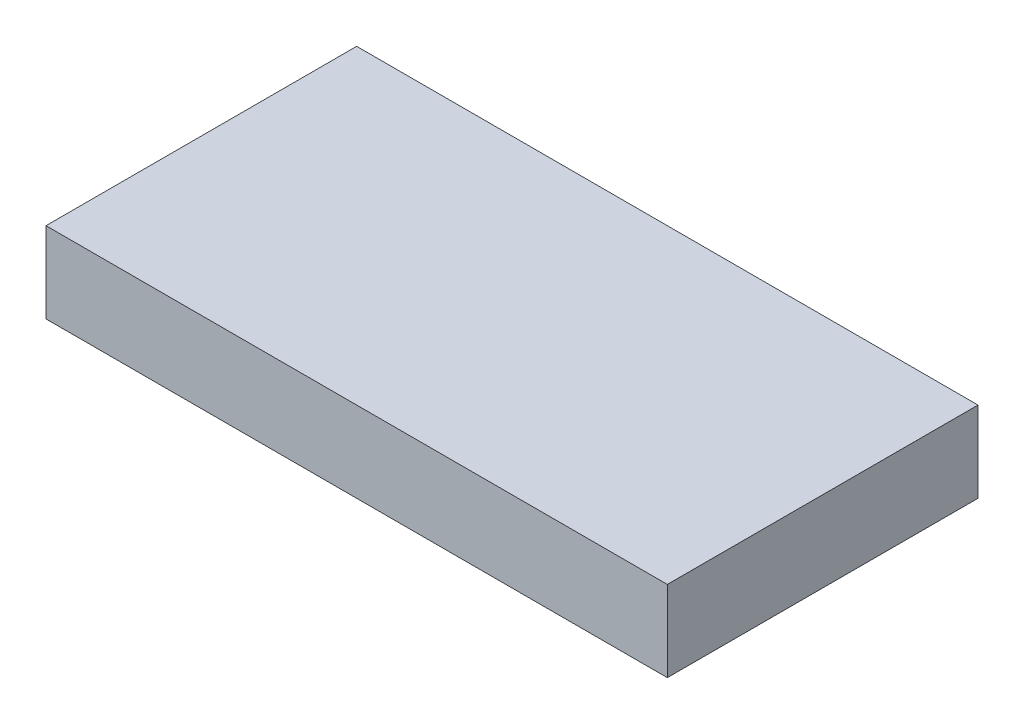
SolidWorks part; units mm, degrees
ref_plane "Front Plane" through (0, 0, 0) normal (0, 0, 1) x (1, 0, 0)
ref_plane "Top Plane" through (0, 0, 0) normal (0, 1, 0) x (1, 0, 0)
ref_plane "Right Plane" through (0, 0, 0) normal (1, 0, 0) x (0, 0, -1)
sketch "Sketch1" plane through (0, 0, 0) normal (0, 1, 0) x (1, 0, 0)
  line L1 (-10, 5) -> (10, 5)
  line L2 (-10, 5) -> (-10, -5)
  line L3 (-10, -5) -> (10, -5)
  line L4 (10, 5) -> (10, -5)
  line L5 (-10, 5) -> (10, -5) construction
  line L6 (-10, -5) -> (10, 5) construction
  point P0 (0, 0)
  dimension "D1" = 10
  dimension "D2" = 20
extrude "Boss-Extrude1" add sketch "Sketch1" along normal blind 2.6
